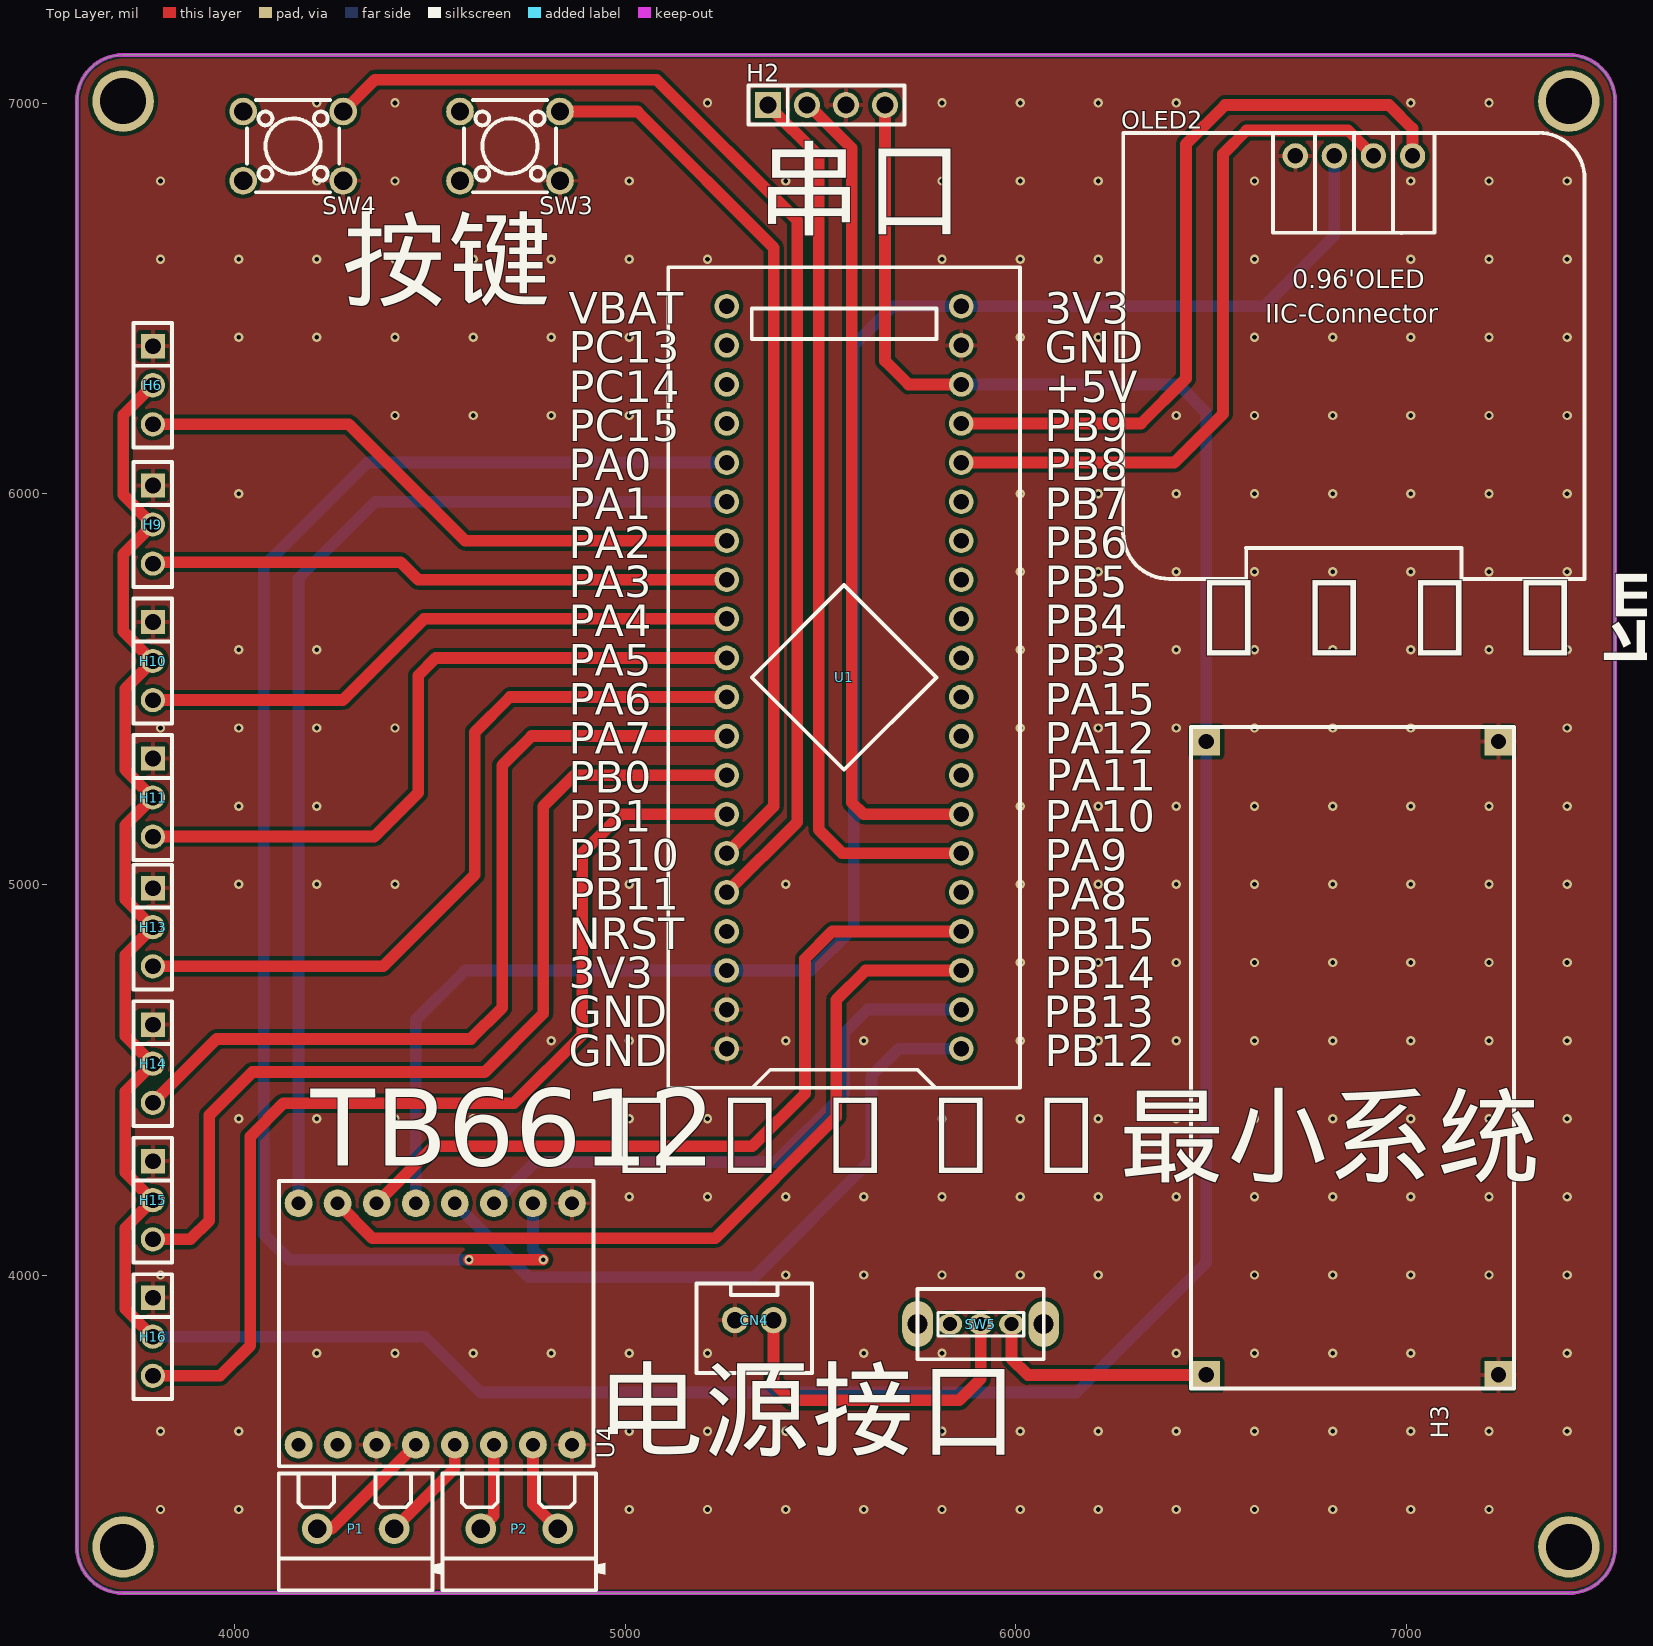
[diagram p0: Top Layer view]
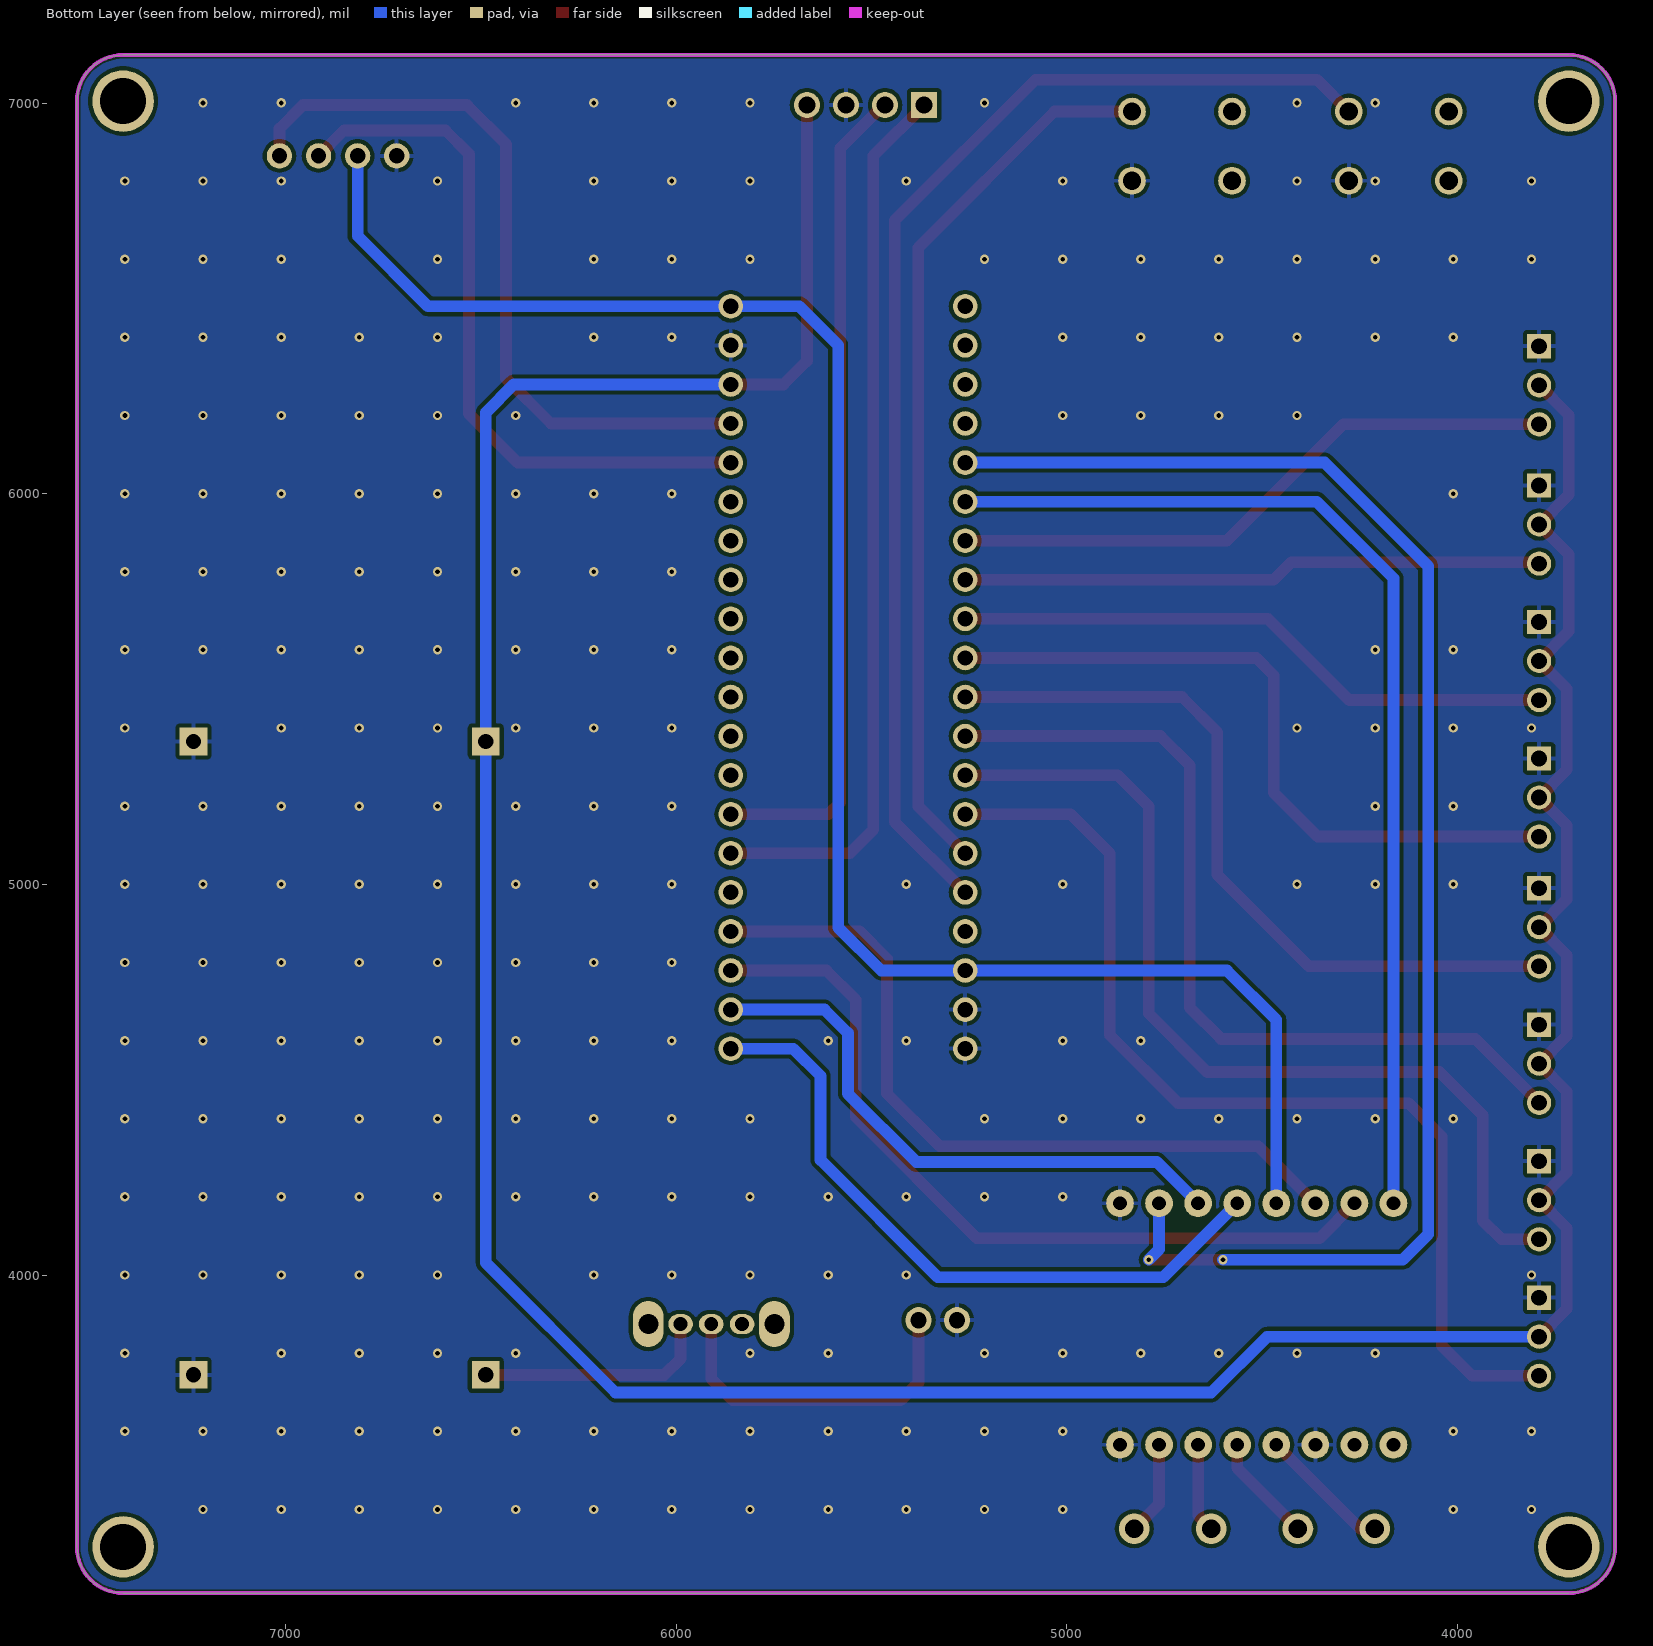
[diagram p1: Bottom Layer view, seen from below]
# Altium PCB MISC52001.pcbdoc
Units mil, origin at the board's own origin, x right, y up, seen from the top; angles counter-clockwise.
Board outline 3937.01 x 3937.01 mil, 2 copper layers (Top Layer, Bottom Layer), stack 62.206 mil thick; 19 components, 44 nets, 115 pads, 224 vias.

## Layer stack, top to bottom
Top Solder Mask Layer: solder mask 0.394, Dk 3.3
Top Layer: signal copper 1.379
Dielectric1: surface 59.449, FR4, Dk 4.5
Bottom Layer: signal copper 1.378
Bottom Solder Mask Layer: solder mask 0.394, Dk 3.3

## Board outline
3714.61,7123.5 ccw(c3714.61,7005.39) 3596.5,7005.39 3596.5,3304.61 ccw(c3714.61,3304.61) 3714.61,3186.5 7415.39,3186.5 ccw(c7415.39,3304.61) 7533.5,3304.61 7533.5,7005.39 ccw(c7415.39,7005.39) 7415.39,7123.5 3714.61,7123.5

## Design rules (kind name [scope] priority, off if disabled: settings)
BoardOutlineClearance copperThickness2oz_1 [All] p2 off: genericclearance=7.99 ignorepadtopadclearanceinfootprint=FALSE except(0: Arc-SplitContinuation Track-SplitContinuation SMDPad-SplitContinuation THPad-SplitContinuation Via-SplitContinuation Fill-SplitContinuation Region-SplitContinuation Poly-SplitContinuation Text-SplitContinuation Hole-SplitContinuation; 5.98: Arc-CutoutEdge Track-CutoutEdge SMDPad-CutoutEdge THPad-CutoutEdge Via-CutoutEdge Text-CutoutEdge; 6.9: Hole-OutlineEdge Hole-CutoutEdge; 10: Poly-OutlineEdge Poly-CutoutEdge; 11.81: Arc-OutlineEdge Track-OutlineEdge SMDPad-OutlineEdge THPad-OutlineEdge Via-OutlineEdge Fill-OutlineEdge Region-OutlineEdge Text-OutlineEdge Fill-CutoutEdge Region-CutoutEdge)
BoardOutlineClearance Plane_innerPlane_1 [All] p4 off: genericclearance=4.02 ignorepadtopadclearanceinfootprint=FALSE except(0: Arc-SplitContinuation Track-SplitContinuation SMDPad-SplitContinuation THPad-SplitContinuation Via-SplitContinuation Fill-SplitContinuation Region-SplitContinuation Poly-SplitContinuation Text-SplitContinuation Hole-SplitContinuation; 5.98: Arc-CutoutEdge Track-CutoutEdge SMDPad-CutoutEdge THPad-CutoutEdge Via-CutoutEdge Text-CutoutEdge; 6.9: Hole-OutlineEdge Hole-CutoutEdge; 10: Poly-OutlineEdge Poly-CutoutEdge; 11.81: Arc-OutlineEdge Track-OutlineEdge SMDPad-OutlineEdge THPad-OutlineEdge Via-OutlineEdge Fill-OutlineEdge Region-OutlineEdge Text-OutlineEdge Fill-CutoutEdge Region-CutoutEdge)
BoardOutlineClearance Copper_copperRegion_1 [All] p6 off: genericclearance=4.02 ignorepadtopadclearanceinfootprint=FALSE except(0: Arc-SplitContinuation Track-SplitContinuation SMDPad-SplitContinuation THPad-SplitContinuation Via-SplitContinuation Fill-SplitContinuation Region-SplitContinuation Poly-SplitContinuation Text-SplitContinuation Hole-SplitContinuation; 5.98: Arc-CutoutEdge Track-CutoutEdge SMDPad-CutoutEdge THPad-CutoutEdge Via-CutoutEdge Text-CutoutEdge; 6.9: Hole-OutlineEdge Hole-CutoutEdge; 10: Poly-OutlineEdge Poly-CutoutEdge; 11.81: Arc-OutlineEdge Track-OutlineEdge SMDPad-OutlineEdge THPad-OutlineEdge Via-OutlineEdge Fill-OutlineEdge Region-OutlineEdge Text-OutlineEdge Fill-CutoutEdge Region-CutoutEdge)
BoardOutlineClearance Copper_copperRegion_copperThickness1oz_1 [All] p8 off: genericclearance=4.02 ignorepadtopadclearanceinfootprint=FALSE except(0: Arc-SplitContinuation Track-SplitContinuation SMDPad-SplitContinuation THPad-SplitContinuation Via-SplitContinuation Fill-SplitContinuation Region-SplitContinuation Poly-SplitContinuation Text-SplitContinuation Hole-SplitContinuation; 5.98: Arc-CutoutEdge Track-CutoutEdge SMDPad-CutoutEdge THPad-CutoutEdge Via-CutoutEdge Text-CutoutEdge; 6.9: Hole-OutlineEdge Hole-CutoutEdge; 10: Poly-OutlineEdge Poly-CutoutEdge; 11.81: Arc-OutlineEdge Track-OutlineEdge SMDPad-OutlineEdge THPad-OutlineEdge Via-OutlineEdge Fill-OutlineEdge Region-OutlineEdge Text-OutlineEdge Fill-CutoutEdge Region-CutoutEdge)
BoardOutlineClearance Copper_copperRegion_Copper_copperRegion_1 [All] p10 off: genericclearance=4.02 ignorepadtopadclearanceinfootprint=FALSE except(0: Arc-SplitContinuation Track-SplitContinuation SMDPad-SplitContinuation THPad-SplitContinuation Via-SplitContinuation Fill-SplitContinuation Region-SplitContinuation Poly-SplitContinuation Text-SplitContinuation Hole-SplitContinuation; 5.98: Arc-CutoutEdge Track-CutoutEdge SMDPad-CutoutEdge THPad-CutoutEdge Via-CutoutEdge Text-CutoutEdge; 6.9: Hole-OutlineEdge Hole-CutoutEdge; 10: Poly-OutlineEdge Poly-CutoutEdge; 11.81: Arc-OutlineEdge Track-OutlineEdge SMDPad-OutlineEdge THPad-OutlineEdge Via-OutlineEdge Fill-OutlineEdge Region-OutlineEdge Text-OutlineEdge Fill-CutoutEdge Region-CutoutEdge)
BoardOutlineClearance copperThickness1oz_1 [All] p12: genericclearance=4.02 ignorepadtopadclearanceinfootprint=FALSE except(0: Arc-SplitContinuation Track-SplitContinuation SMDPad-SplitContinuation THPad-SplitContinuation Via-SplitContinuation Fill-SplitContinuation Region-SplitContinuation Poly-SplitContinuation Text-SplitContinuation Hole-SplitContinuation; 5.98: Arc-CutoutEdge Track-CutoutEdge SMDPad-CutoutEdge THPad-CutoutEdge Via-CutoutEdge Text-CutoutEdge; 6.9: Hole-OutlineEdge Hole-CutoutEdge; 10: Poly-OutlineEdge Poly-CutoutEdge; 11.81: Arc-OutlineEdge Track-OutlineEdge SMDPad-OutlineEdge THPad-OutlineEdge Via-OutlineEdge Fill-OutlineEdge Region-OutlineEdge Text-OutlineEdge Fill-CutoutEdge Region-CutoutEdge)
Clearance copperThickness2oz [All] p1 off: gap=7.99 ignorepadtopadclearanceinfootprint=FALSE except(5.98: SMDPad-Track SMDPad-SMDPad THPad-Track SMDPad-THPad THPad-THPad Track-Via SMDPad-Via THPad-Via Via-Via Fill-SMDPad Region-SMDPad Fill-THPad Region-THPad Fill-Via Region-Via Fill-Fill Fill-Region Region-Region Arc-Track Arc-SMDPad Arc-THPad Arc-Via Fill-Arc Region-Arc Arc-Arc Text-Track SMDPad-Text Text-THPad Text-Via Fill-Text Region-Text Arc-Text Text-Text; 6.9: Hole-Track Hole-SMDPad Hole-THPad Hole-Via Fill-Hole Region-Hole Hole-Arc Hole-Text; 10: Poly-Track Poly-SMDPad Poly-THPad Poly-Via Poly-Fill Poly-Region Poly-Poly Poly-Arc Poly-Text Poly-Hole; 11.81: Fill-Track Region-Track)
Clearance Plane_innerPlane [All] p3 off: gap=4.02 ignorepadtopadclearanceinfootprint=FALSE except(5.98: SMDPad-Track SMDPad-SMDPad THPad-Track SMDPad-THPad THPad-THPad Track-Via SMDPad-Via THPad-Via Via-Via Fill-SMDPad Region-SMDPad Fill-THPad Region-THPad Fill-Via Region-Via Fill-Fill Fill-Region Region-Region Arc-Track Arc-SMDPad Arc-THPad Arc-Via Fill-Arc Region-Arc Arc-Arc Text-Track SMDPad-Text Text-THPad Text-Via Fill-Text Region-Text Arc-Text Text-Text; 6.9: Hole-Track Hole-SMDPad Hole-THPad Hole-Via Fill-Hole Region-Hole Hole-Arc Hole-Text; 10: Poly-Track Poly-SMDPad Poly-THPad Poly-Via Poly-Fill Poly-Region Poly-Poly Poly-Arc Poly-Text Poly-Hole; 11.81: Fill-Track Region-Track)
Clearance Copper_copperRegion [All] p5 off: gap=4.02 ignorepadtopadclearanceinfootprint=FALSE except(5.98: SMDPad-Track SMDPad-SMDPad THPad-Track SMDPad-THPad THPad-THPad Track-Via SMDPad-Via THPad-Via Via-Via Fill-SMDPad Region-SMDPad Fill-THPad Region-THPad Fill-Via Region-Via Fill-Fill Fill-Region Region-Region Arc-Track Arc-SMDPad Arc-THPad Arc-Via Fill-Arc Region-Arc Arc-Arc Text-Track SMDPad-Text Text-THPad Text-Via Fill-Text Region-Text Arc-Text Text-Text; 6.9: Hole-Track Hole-SMDPad Hole-THPad Hole-Via Fill-Hole Region-Hole Hole-Arc Hole-Text; 10: Poly-Track Poly-SMDPad Poly-THPad Poly-Via Poly-Fill Poly-Region Poly-Poly Poly-Arc Poly-Text Poly-Hole; 11.81: Fill-Track Region-Track)
Clearance Copper_copperRegion_copperThickness1oz [All] p7 off: gap=4.02 ignorepadtopadclearanceinfootprint=FALSE except(5.98: SMDPad-Track SMDPad-SMDPad THPad-Track SMDPad-THPad THPad-THPad Track-Via SMDPad-Via THPad-Via Via-Via Fill-SMDPad Region-SMDPad Fill-THPad Region-THPad Fill-Via Region-Via Fill-Fill Fill-Region Region-Region Arc-Track Arc-SMDPad Arc-THPad Arc-Via Fill-Arc Region-Arc Arc-Arc Text-Track SMDPad-Text Text-THPad Text-Via Fill-Text Region-Text Arc-Text Text-Text; 6.9: Hole-Track Hole-SMDPad Hole-THPad Hole-Via Fill-Hole Region-Hole Hole-Arc Hole-Text; 10: Poly-Track Poly-SMDPad Poly-THPad Poly-Via Poly-Fill Poly-Region Poly-Poly Poly-Arc Poly-Text Poly-Hole; 11.81: Fill-Track Region-Track)
Clearance Copper_copperRegion_Copper_copperRegion [All] p9 off: gap=4.02 ignorepadtopadclearanceinfootprint=FALSE except(5.98: SMDPad-Track SMDPad-SMDPad THPad-Track SMDPad-THPad THPad-THPad Track-Via SMDPad-Via THPad-Via Via-Via Fill-SMDPad Region-SMDPad Fill-THPad Region-THPad Fill-Via Region-Via Fill-Fill Fill-Region Region-Region Arc-Track Arc-SMDPad Arc-THPad Arc-Via Fill-Arc Region-Arc Arc-Arc Text-Track SMDPad-Text Text-THPad Text-Via Fill-Text Region-Text Arc-Text Text-Text; 6.9: Hole-Track Hole-SMDPad Hole-THPad Hole-Via Fill-Hole Region-Hole Hole-Arc Hole-Text; 10: Poly-Track Poly-SMDPad Poly-THPad Poly-Via Poly-Fill Poly-Region Poly-Poly Poly-Arc Poly-Text Poly-Hole; 11.81: Fill-Track Region-Track)
Clearance copperThickness1oz [All] p11: gap=4.02 ignorepadtopadclearanceinfootprint=FALSE except(5.98: SMDPad-Track SMDPad-SMDPad THPad-Track SMDPad-THPad THPad-THPad Track-Via SMDPad-Via THPad-Via Via-Via Fill-SMDPad Region-SMDPad Fill-THPad Region-THPad Fill-Via Region-Via Fill-Fill Fill-Region Region-Region Arc-Track Arc-SMDPad Arc-THPad Arc-Via Fill-Arc Region-Arc Arc-Arc Text-Track SMDPad-Text Text-THPad Text-Via Fill-Text Region-Text Arc-Text Text-Text; 6.9: Hole-Track Hole-SMDPad Hole-THPad Hole-Via Fill-Hole Region-Hole Hole-Arc Hole-Text; 10: Poly-Track Poly-SMDPad Poly-THPad Poly-Via Poly-Fill Poly-Region Poly-Poly Poly-Arc Poly-Text Poly-Hole; 11.81: Fill-Track Region-Track)
DiffPairsRouting differentialPair [All] p1: maxlimit=6 minlimit=6 mostfreqgap=6 toplayer_minwidth=5 toplayer_prefwidth=10 toplayer_maxwidth=100 toplayer_mingap=6 toplayer_prefgap=6 toplayer_maxgap=6 bottomlayer_minwidth=5 bottomlayer_prefwidth=10 bottomlayer_maxwidth=100 bottomlayer_mingap=6 bottomlayer_prefgap=6 bottomlayer_maxgap=6 maxuncoupledlength=10
HoleToHoleClearance otherClearance [All] p1: gap=11.81 allowstackedmicrovias=TRUE
Length netLength [All] p1: minlimit=0 maxlimit=0
PasteMaskExpansion pasteMaskExpansion [All] p1: expansion=0
PlaneConnect innerPlane [All] p1: planeconnectstyle=Relief reliefexpansion=20 reliefentries=4 reliefconductorwidth=10 reliefairgap=10
PolygonConnect copperRegion_copperThickness1oz [All] p1 off: connectstyle=Relief reliefconductorwidth=10 reliefentries=4 polygonreliefangle="90 Angle" airgapwidth=10 via.connectstyle=Relief via.reliefconductorwidth=10 via.reliefentries=4 via.polygonreliefangle="90 Angle" via.airgapwidth=10
PolygonConnect copperRegion_Copper_copperRegion [All] p2 off: connectstyle=Relief reliefconductorwidth=10 reliefentries=4 polygonreliefangle="90 Angle" airgapwidth=10 via.connectstyle=Relief via.reliefconductorwidth=10 via.reliefentries=4 via.polygonreliefangle="90 Angle" via.airgapwidth=10
PolygonConnect copperRegion [All] p3: connectstyle=Relief reliefconductorwidth=10 reliefentries=4 polygonreliefangle="90 Angle" airgapwidth=10 via.connectstyle=Relief via.reliefconductorwidth=10 via.reliefentries=4 via.polygonreliefangle="90 Angle" via.airgapwidth=10
RoutingVias viaSize [All] p1: holewidth=12.01 width=24.02 viastyle="Through Hole" minholewidth=11.81 minwidth=19.68 maxholewidth=248.03 maxwidth=393.7
SolderMaskExpansion solderMaskExpansion [IsVia] p1: expansion=-1000 istentingtop=TRUE
SolderMaskExpansion solderMaskExpansion [All] p2: expansion=2 istentingtop=FALSE
Width copperThickness2oz_2 [All] p1 off: maxlimit=100 minlimit=8 preferedwidth=10
Width copperThickness1oz_2 [All] p2: maxlimit=100 minlimit=5 preferedwidth=10

## Components (designator, comment, footprint, x,y, rotation, side; value= is the part's Value field where it differs from the comment)
CN4 "XH2.54*2P_直插" CONN-TH_2P-P2.50-XH2.54-2P 5330,3885 r0 top
H2 "" HDR-TH_4P-P2.54-V-M 5515,6995 r0 top
H3 "" HDR-TH_4P-P2.54-V-F-R2-C2-S2.54 7235,3745 r90 top
H6 "" HDR-TH_3P-P2.54-V-F 3791.07,6277.96 r270 top
H9 "" HDR-TH_3P-P2.54-V-F 3791.07,5921.47 r270 top
H10 "" HDR-TH_3P-P2.54-V-F 3791.07,5572.1 r270 top
H11 "" HDR-TH_3P-P2.54-V-F 3791.07,5222.73 r270 top
H13 "" HDR-TH_3P-P2.54-V-F 3791.07,4890.83 r270 top
H14 "" HDR-TH_3P-P2.54-V-F 3791.07,4541.47 r270 top
H15 "" HDR-TH_3P-P2.54-V-F 3791.07,4192.1 r270 top
H16 "" HDR-TH_3P-P2.54-V-F 3791.07,3842.73 r270 top
OLED2 "" 0.96OLED_4P 6865,6865 r0 top
P1 "KF301-2P接线端子" CONN-TH_XY301V-A-5.0-2P 4310.04,3351.24 r0 top
P2 "KF301-2P接线端子" CONN-TH_XY301V-A-5.0-2P 4728.76,3351.24 r0 top
SW3 "" SW-TH_4P-L6.0-W6.0-P4.50-LS6.5 4705,6890 r180 top
SW4 "" SW-TH_4P-L6.0-W6.0-P4.50-LS6.5 4150,6890 r180 top
SW5 "" 拨动开关 5915,3875 r180 top
U1 "STM32F103C8T6-Card" CONN-TH_L53.3-W22.9_STM32F103C8T6-CARD 5560,5530 r90 top
U4 "" tb6612 4163.76,3566.24 r90 top

## Footprints (in the part's own frame and the unit in brackets; to place one, negate y for a bottom-side part, rotate by r counter-clockwise, add the part's x,y. Pads: shape width x height; smd on the part's side, far side on the other; paste and mask are expansions set on the pad)
0.96OLED_4P [mm]
  round 1.65 hole 1 copper offset 0,0: 1(-3.81,-0.001) 2(-1.27,0.002) 3(1.27,0.002) 4(3.81,0.002)
  silkscreen extent -15,-27.5 15,1.5
CONN-TH_2P-P2.50-XH2.54-2P [mm]
  round 1.7 hole 1.05 paste+0 mask+0.05: 1(1.25,0) 2(-1.25,0)
  silkscreen extent -3.75,-3.42 3.75,2.37
CONN-TH_L53.3-W22.9_STM32F103C8T6-CARD [mm]
  round 1.6 hole 1: 1(-24.13,-7.62) 2(-21.59,-7.62) 3(-19.05,-7.62) 4(-16.51,-7.62) 5(-13.97,-7.62) 6(-11.43,-7.62) 7(-8.89,-7.62) 8(-6.35,-7.62) 9(-3.81,-7.62) 10(-1.27,-7.62) 11(1.27,-7.62) 12(3.81,-7.62) 13(6.35,-7.62) 14(8.89,-7.62) 15(11.43,-7.62) 16(13.97,-7.62) 17(16.51,-7.62) 18(19.05,-7.62) 19(21.59,-7.62) 20(24.13,-7.62) 21(24.13,7.62) 22(21.59,7.62) 23(19.05,7.62) 24(16.51,7.62) 25(13.97,7.62) 26(11.43,7.62) 27(8.89,7.62) 28(6.35,7.62) 29(3.81,7.62) 30(1.27,7.62) 31(-1.27,7.62) 32(-3.81,7.62) 33(-6.35,7.62) 34(-8.89,7.62) 35(-11.43,7.62) 36(-13.97,7.62) 37(-16.51,7.62) 38(-19.05,7.62) 39(-21.59,7.62) 40(-24.13,7.62)
  silkscreen extent -26.67,-11.43 26.67,11.43
CONN-TH_XY301V-A-5.0-2P [mm]
  round 2 hole 1.2: 1(-2.5,0) 2(2.5,0)
  silkscreen extent -5,-4 5.6,3.6
HDR-TH_3P-P2.54-V-F [mil]
  rect 62x62 hole 40.16: 1(-100,0)
  round 62 hole 40.16: 2(0,0) 3(100,0)
  silkscreen extent -160,-49 160,49
HDR-TH_4P-P2.54-V-F-R2-C2-S2.54 [mm]
  rect 1.8x1.8 hole 1: 1(0,19) 2(41.174,19) 3(0,0) 4(41.174,0)
  silkscreen extent -0.88,-1.01 42.12,19.99
HDR-TH_4P-P2.54-V-M [mm]
  rect 1.7x1.7 hole 1.1: 1(-3.81,0)
  round 1.7 hole 1.1: 2(-1.27,0) 3(1.27,0) 4(3.81,0)
  silkscreen extent -5.08,-1.27 5.08,1.27
SW-TH_4P-L6.0-W6.0-P4.50-LS6.5 [mm]
  round 1.8 hole 1.2: 1(-3.25,2.25) 2(3.25,2.25) 3(-3.25,-2.25) 4(3.25,-2.25)
  silkscreen extent -3,-3 3,3
tb6612 [mm]
  round 1.8 hole 0.9: 1(0,0) 2(0,-2.54) 3(0,-5.08) 4(0,-7.62) 5(0,-10.16) 6(0,-12.7) 7(0,-15.24) 8(0,-17.78) 9(15.697,-17.78) 10(15.697,-15.24) 11(15.697,-12.7) 12(15.697,-10.16) 13(15.697,-7.62) 14(15.697,-5.08) 15(15.697,-2.54) 16(15.697,0)
  silkscreen extent -1.4,-19.18 17.14,1.27
拨动开关 [mil]
  oval 63x51.2 hole 35.4 paste+0 mask+2: 1(-73.4,0) 2(5,0) 3(84,0)
  oval 78.7x118.1 hole 51.2 paste+0 mask+2: 4(166.7,0) 5(-156.1,0)
  silkscreen extent -156,-90 167,90

## Free pads (board coordinates)
  round 157.48 hole 118.11: 1(3714.61,7005.39) 1(3714.61,3304.61) 1(7415.39,7005.39) 1(7415.39,3304.61)

## Via types
v1: diameter 24.02, hole 12, Top Layer to Bottom Layer, 224 vias

## Nets (pads, with @x,y where several pads share a name; then routed paths per layer and width w, separated by ;. In a path a pad name is that pad's centre, name@x,y a point inside that pad or via, vN(x,y) a via of type N, cw(c..) or ccw(c..) an arc to the next point about the centre after c; other vN are vias at no path point)
12V: H3.1 SW5.1 | length 604.2
  Top Layer w30: SW5.1 5988.4,3786.6 6030,3745 H3.1
$1N17118: CN4.1 SW5.2 | length 871.7
  Top Layer w30: CN4.1 5379.22,3725.78 5425,3680 5855,3680 5910,3735 SW5.2
$1N17171: P1.1 U4.4 | length 341.2
  Top Layer w30: P1.1 4248.76,3351.24 U4.4
$1N17172: P1.2 U4.5 | length 279.3
  Top Layer w30: P1.2 4563.76,3506.54 U4.5
$1N17173: P2.1 U4.6 | length 228.8
  Top Layer w30: P2.1 4663.76,3384.67 U4.6
$1N17174: P2.2 U4.7 | length 241.3
  Top Layer w30: U4.7 4763.76,3414.67 P2.2
+5V: H2.4 H3.2 H6.2 H9.2 H10.2 H11.2 H13.2 H14.2 H15.2 H16.2 U1.18 | length 9455.9
  Top Layer w30: H16.2 3720,3913.8 3720,4121.03 H15.2 3720,4263.17 3720,4470.4 H14.2 3720,4612.54 3720,4819.77 H13.2 3720,4961.9 3720,5151.66 H11.2 3720,5293.8 3720,5501.03 H10.2 3715,5648.17 3715,5845.4 H9.2 3715,5997.54 3715,6201.89 H6.2 ; H2.4 5665,6340 5725,6280 U1.18
  Bottom Layer w30: H16.2 4487.27,3842.73 4630,3700 6155,3700 6486.97,4031.97 H3.2 6486.97,6208.03 6415,6280 U1.18
+12V: U4.1
GND: CN4.2 H2.3 H3.3 H3.4 H6.1 H9.1 H10.1 H11.1 H13.1 H14.1 H15.1 H16.1 OLED2.1 SW3.1 SW4.1 U1.19 U1.39 U1.40 U4.3 U4.8 U4.9
  other v1: 3810.6,3400.6 4010.6,3400.6 5010.6,3400.6 5210.6,3400.6 5410.6,3400.6 5610.6,3400.6 5810.6,3400.6 6010.6,3400.6 6210.6,3400.6 6410.6,3400.6 6610.6,3400.6 6810.6,3400.6 7010.6,3400.6 7210.6,3400.6 3810.6,3600.6 4010.6,3600.6 5010.6,3600.6 5210.6,3600.6 5410.6,3600.6 5610.6,3600.6 5810.6,3600.6 6010.6,3600.6 6210.6,3600.6 6410.6,3600.6 6610.6,3600.6 6810.6,3600.6 7010.6,3600.6 7210.6,3600.6 7410.6,3600.6 4210.6,3800.6 4410.6,3800.6 4610.6,3800.6 4810.6,3800.6 5010.6,3800.6 5210.6,3800.6 5610.6,3800.6 5810.6,3800.6 6410.6,3800.6 6610.6,3800.6 6810.6,3800.6 7010.6,3800.6 7410.6,3800.6 3810.6,4000.6 5410.6,4000.6 5610.6,4000.6 5810.6,4000.6 6010.6,4000.6 6210.6,4000.6 6610.6,4000.6 6810.6,4000.6 7010.6,4000.6 7210.6,4000.6 7410.6,4000.6 5010.6,4200.6 5210.6,4200.6 5410.6,4200.6 5610.6,4200.6 5810.6,4200.6 6010.6,4200.6 6210.6,4200.6 6410.6,4200.6 6610.6,4200.6 6810.6,4200.6 7010.6,4200.6 7210.6,4200.6 7410.6,4200.6 4010.6,4400.6 4210.6,4400.6 4410.6,4400.6 4610.6,4400.6 4810.6,4400.6 5010.6,4400.6 5210.6,4400.6 5810.6,4400.6 6010.6,4400.6 6210.6,4400.6 6410.6,4400.6 6610.6,4400.6 6810.6,4400.6 7010.6,4400.6 7210.6,4400.6 7410.6,4400.6 4810.6,4600.6 5010.6,4600.6 5410.6,4600.6 5610.6,4600.6 6010.6,4600.6 6210.6,4600.6 6410.6,4600.6 6610.6,4600.6 6810.6,4600.6 7010.6,4600.6 7210.6,4600.6 7410.6,4600.6 6010.6,4800.6 6210.6,4800.6 6410.6,4800.6 6610.6,4800.6 6810.6,4800.6 7010.6,4800.6 7210.6,4800.6 7410.6,4800.6 4010.6,5000.6 4210.6,5000.6 4410.6,5000.6 5010.6,5000.6 5410.6,5000.6 6010.6,5000.6 6210.6,5000.6 6410.6,5000.6 6610.6,5000.6 6810.6,5000.6 7010.6,5000.6 7210.6,5000.6 7410.6,5000.6 4010.6,5200.6 4210.6,5200.6 6010.6,5200.6 6210.6,5200.6 6410.6,5200.6 6610.6,5200.6 6810.6,5200.6 7010.6,5200.6 7210.6,5200.6 7410.6,5200.6 3810.6,5400.6 4010.6,5400.6 4210.6,5400.6 4410.6,5400.6 6010.6,5400.6 6210.6,5400.6 6410.6,5400.6 6610.6,5400.6 6810.6,5400.6 7010.6,5400.6 7410.6,5400.6 4010.6,5600.6 4210.6,5600.6 6010.6,5600.6 6210.6,5600.6 6410.6,5600.6 6610.6,5600.6 6810.6,5600.6 7010.6,5600.6 7210.6,5600.6 7410.6,5600.6 6010.6,5800.6 6210.6,5800.6 6410.6,5800.6 6610.6,5800.6 6810.6,5800.6 7010.6,5800.6 7210.6,5800.6 7410.6,5800.6 4010.6,6000.6 6010.6,6000.6 6210.6,6000.6 6410.6,6000.6 6610.6,6000.6 6810.6,6000.6 7010.6,6000.6 7210.6,6000.6 7410.6,6000.6 4410.6,6200.6 4610.6,6200.6 4810.6,6200.6 5010.6,6200.6 6410.6,6200.6 6610.6,6200.6 6810.6,6200.6 7010.6,6200.6 7210.6,6200.6 7410.6,6200.6 4010.6,6400.6 4210.6,6400.6 4410.6,6400.6 4610.6,6400.6 4810.6,6400.6 5010.6,6400.6 6010.6,6400.6 6210.6,6400.6 6610.6,6400.6 6810.6,6400.6 7010.6,6400.6 7210.6,6400.6 7410.6,6400.6 3810.6,6600.6 4010.6,6600.6 4210.6,6600.6 4410.6,6600.6 4610.6,6600.6 4810.6,6600.6 5010.6,6600.6 5210.6,6600.6 5810.6,6600.6 6010.6,6600.6 6210.6,6600.6 6610.6,6600.6 7010.6,6600.6 7210.6,6600.6 7410.6,6600.6 3810.6,6800.6 4210.6,6800.6 4410.6,6800.6 5010.6,6800.6 5410.6,6800.6 5810.6,6800.6 6010.6,6800.6 6210.6,6800.6 6610.6,6800.6 7010.6,6800.6 7210.6,6800.6 7410.6,6800.6 4210.6,7000.6 4410.6,7000.6 5210.6,7000.6 5810.6,7000.6 6010.6,7000.6 6210.6,7000.6 6410.6,7000.6 7010.6,7000.6 7210.6,7000.6
NRST: U1.37
PA0: U1.25 U4.10 | length 3901.8
  Top Layer w30: v1(4600,4040) v1(4790,4040)
  Bottom Layer w30: v1(4600,4040) 4140,4040 4075,4105 4075,5815 4340,6080 U1.25 ; U4.10 4763.76,4066.24 v1(4790,4040)
PA1: U1.26 U4.16 | length 2777
  Bottom Layer w30: U4.16 4163.76,5783.76 4360,5980 U1.26
PA2: H6.3 U1.27 | length 1592.3
  Top Layer w30: H6.3 4292.04,6177.96 4590,5880 U1.27
PA3: H9.3 U1.28 | length 1489
  Top Layer w30: H9.3 3794.6,5825 4425,5825 4470,5780 U1.28
PA4: H10.3 U1.29 | length 1555
  Top Layer w30: H10.3 4277.1,5472.1 4485,5680 U1.29
PA5: H11.3 U1.30 | length 1834.1
  Top Layer w30: H11.3 4357.73,5122.73 4470,5235 4470,5535 4515,5580 U1.30
PA6: H13.3 U1.31 | length 1968.2
  Top Layer w30: H13.3 4380.83,4790.83 4615,5025 4615,5390 4705,5480 U1.31
PA7: H14.3 U1.32 | length 2220.9
  Top Layer w30: H14.3 3954.6,4605 4605,4605 4685,4685 4685,5305 4760,5380 U1.32
PA8: U1.5
PA9: H2.1 U1.6 | length 2298.7
  Top Layer w30: H2.1 5495,6865 5495,5140 5555,5080 U1.6
PA10: H2.2 U1.7 | length 2130.1
  Top Layer w30: H2.2@5465,7000 5580,6885 5580,5210 5610,5180 U1.7
PA11: U1.8
PA12: U1.9
PA15: U1.10
PB0: H15.3 U1.33 | length 2429.6
  Top Layer w30: H15.3 3887.1,4092.1 3935,4140 3935,4410 4045,4520 4640,4520 4790,4670 4790,5200 4870,5280 U1.33
PB1: H16.3 U1.34 | length 2650.1
  Top Layer w30: H16.3 3962.73,3742.73 4040,3820 4040,4355 4125,4440 4715,4440 4890,4615 4890,5080 4990,5180 U1.34
PB3: U1.11
PB4: U1.12
PB5: U1.13
PB6: U1.14
PB7: U1.15
PB8: OLED2.3 U1.16 | length 1823.5
  Top Layer w30: U1.16 6405,6080 6530,6205 6530,6870 6590,6930 6850.05,6930 OLED2.3@6915,6865.05
PB9: OLED2.4 U1.17 | length 1938.9
  Top Layer w30: U1.17 6320,6180 6435,6295 6435,6895 6535,6995 6955,6995 7015,6935 OLED2.4@7015,6865.05
PB10: SW3.3 U1.35 | length 2291.1
  Top Layer w30: SW3.3 5031.42,6978.58 5380,6630 5380,5200 U1.35
PB11: SW4.3 U1.36 | length 3139.4
  Top Layer w30: SW4.3 4359.37,7060 5080,7060 5440,6700 5440,5160 U1.36
PB12: U1.1 U4.12 | length 1742.9
  Bottom Layer w30: U4.12 4753,3995 5330,3995 5630,4295 5630,4510 5700,4580 U1.1
PB13: U1.2 U4.11 | length 1492.4
  Bottom Layer w30: U4.11 4769.52,4290 5385,4290 5560,4465 5560,4620 5620,4680 U1.2
PB14: U1.3 U4.15 | length 2092.7
  Top Layer w30: U4.15 4353,4095 5230,4095 5540,4405 5540,4705 5615,4780 U1.3
PB15: U1.4 U4.14 | length 1986.5
  Top Layer w30: U4.14 4509.52,4330 5325,4330 5460,4465 5460,4810 5530,4880 U1.4
PC13: U1.22
PC14: U1.23
PC15: U1.24
VBAT: U1.21
VCC: OLED2.2 U1.20 U1.38 U4.13 | length 4729.6
  Bottom Layer w30: U4.13 4463.76,4653.76 4590,4780 U1.38 5475,4780 5585,4890 5585,6380 5685,6480 U1.20 6635,6480 6815,6660 OLED2.2@6815,6865.05
pads on no net: SW3.2 SW3.4 SW4.2 SW4.4 SW5.3 SW5.4 SW5.5 U4.2

## Polygon pours and split planes (outlines as drawn)
GND on Bottom Layer (solid, remove dead copper, pour order 2): 3525,7245 3525,3080 7700,3080 7700,7245
GND on Top Layer (solid, remove dead copper, pour order 2): 3000,7415 3000,3000 7930,3000 7930,7415

## Keep-outs
Board Outline Layer:
  the board outline again, w10

## Silkscreen, mask and mechanical layers (free items; w line width, h text height)
Top Silkscreen Layer:
  text "串口" at 5335,6685 h196.85
  text "按键" at 4275,6505 h196.85
  text "VBAT" at 4855.95,6435 h80
  text "3V3" at 6074.16,6435 h80
  text "PC13" at 4855.95,6335 h80
  text "GND" at 6074.16,6335 h80
  text "PC14" at 4855.95,6235 h80
  text "+5V" at 6074.16,6235 h80
  text "PC15" at 4855.95,6135 h80
  text "PB9" at 6074.16,6135 h80
  text "PA0" at 4855.95,6035 h80
  text "PB8" at 6074.16,6035 h80
  text "PA1" at 4855.95,5935 h80
  text "PB7" at 6074.16,5935 h80
  text "PA2" at 4855.95,5835 h80
  text "PB6" at 6074.16,5835 h80
  text "PA3" at 4855.95,5735 h80
  text "PB5" at 6074.16,5735 h80
  text "PA4" at 4855.95,5635 h80
  text "PB4" at 6074.16,5635 h80
  text "Oled显示器" at 6410,5585 h196.85
  text "PA5" at 4855.95,5535 h80
  text "PB3" at 6074.16,5535 h80
  text "PA6" at 4855.95,5435 h80
  text "PA15" at 6074.16,5435 h80
  text "PA7" at 4855.95,5335 h80
  text "PA12" at 6074.16,5335 h80
  text "PA11" at 6075.95,5240 h80
  text "PB0" at 4855.95,5235 h80
  text "PB1" at 4855.95,5135 h80
  text "PA10" at 6074.16,5135 h80
  text "PB10" at 4855.95,5035 h80
  text "PA9" at 6074.16,5035 h80
  text "PB11" at 4855.95,4935 h80
  text "PA8" at 6074.16,4935 h80
  text "NRST" at 4855.95,4835 h80
  text "PB15" at 6074.16,4835 h80
  text "3V3" at 4855.95,4735 h80
  text "PB14" at 6074.16,4735 h80
  text "GND" at 4855.95,4635 h80
  text "PB13" at 6070.95,4635 h80
  text "GND" at 4855.95,4535 h80
  text "PB12" at 6074.16,4535 h80
  text "TB6612" at 4195,4280 h196.85
  text "STM32最小系统" at 4914.45,4261.57 h196.85
  text "电源接口" at 4932.87,3561.57 h196.85